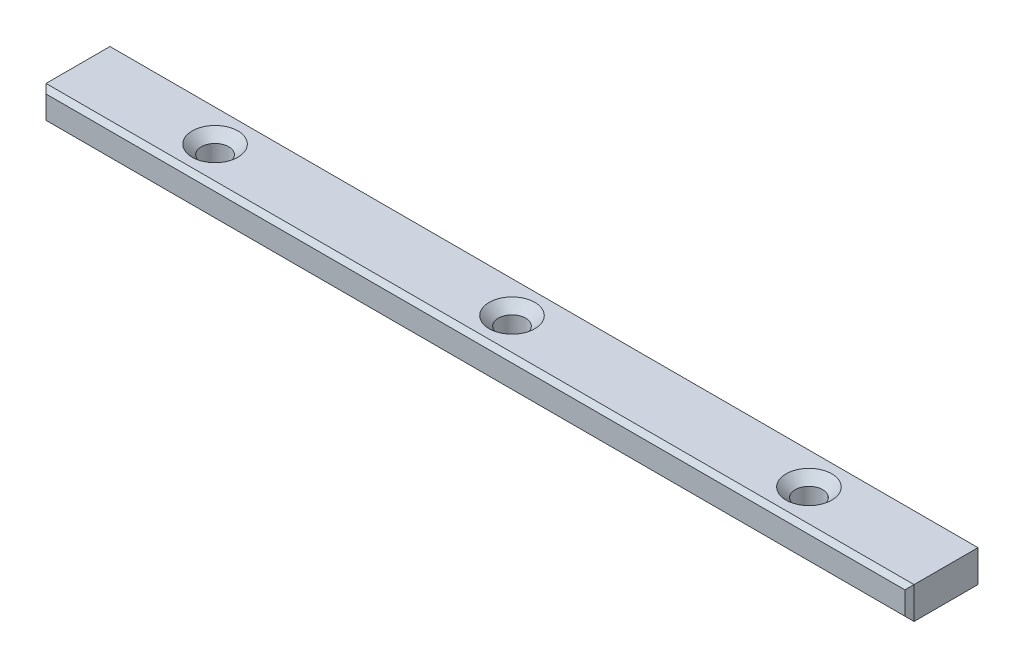
from build123d import *

# Parameters (mm, degrees)
SKETCH1_W           = 190
SKETCH1_H           = 16
BOSS_EXTRUDE1_DEPTH = 3.5
HOLE1_D             = 6
HOLE1_DEPTH         = 20
HOLE1_CSINK_D       = 10
HOLE1_CSINK_ANGLE   = 90
CHAMFER1_SIZE       = 1


with BuildPart() as part:
    # Sketch1 → Boss-Extrude1 (new, symmetric)
    with BuildSketch(Plane(origin=(0, 0, 0), x_dir=(1, 0, 0), z_dir=(0, 1, 0))):
        Rectangle(SKETCH1_W, SKETCH1_H)
    extrude(amount=BOSS_EXTRUDE1_DEPTH, both=True)

    # Hole1
    with Locations(Plane(origin=(0, 3.5, 0), x_dir=(1, 0, 0), z_dir=(0, 1, 0))):
        with Locations((-65, 0), (0, 0), (65, 0)):
            CounterSinkHole(HOLE1_D / 2, HOLE1_CSINK_D / 2, depth=HOLE1_DEPTH, counter_sink_angle=HOLE1_CSINK_ANGLE)

    # Chamfer1
    chamfer1_edges = [part.edges().sort_by_distance(p)[0] for p in [
        (0, 3.5, 8),
        (0, -3.5, 8),
        (0, -3.5, -8),
        (95, 0, 8),
        (-95, 0, 8),
        (-95, 0, -8),
        (95, 0, -8),
        (0, 3.5, -8),
    ]]
    chamfer(chamfer1_edges, length=CHAMFER1_SIZE)


solid = part.part
